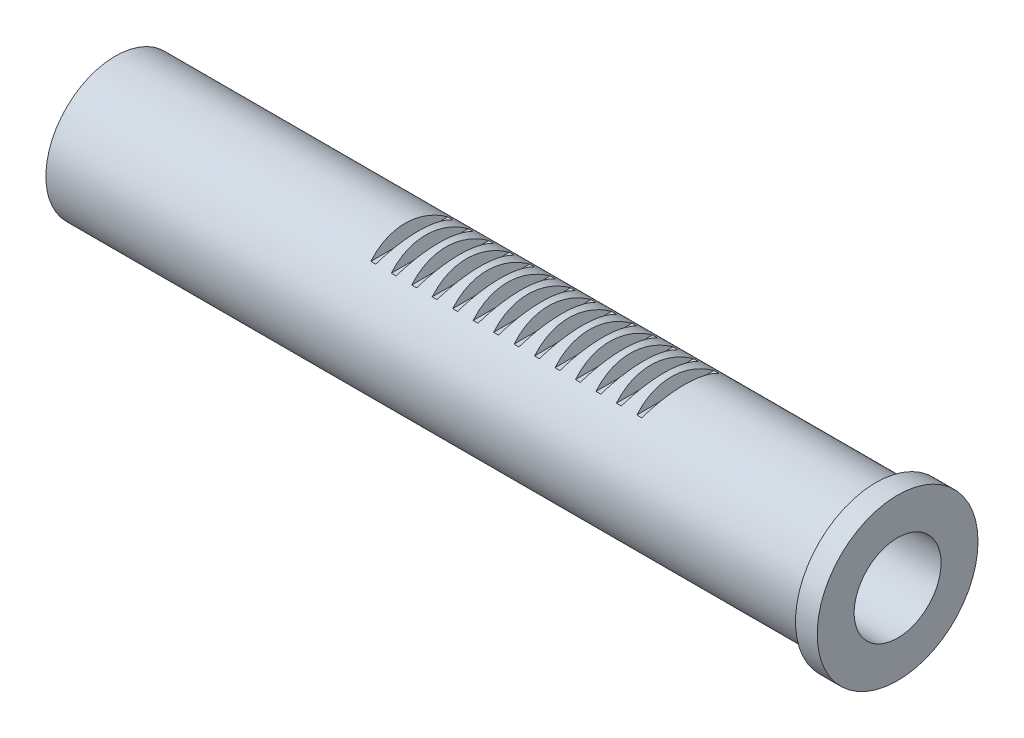
from build123d import *

# Parameters (mm, degrees)
SKETCH1_R               = 16
BOSS_EXTRUDE1_DEPTH     = 175
SKETCH2_R               = 18.5
BOSS_EXTRUDE2_DEPTH     = 5
SKETCH3_R               = 10
CUT_EXTRUDE1_DEPTH      = 100
SKETCH4_R               = 6
CUT_EXTRUDE2_DEPTH      = 8000
CUT_EXTRUDE3_DEPTH      = 182.891451146
CUT_EXTRUDE3_DEPTH_BACK = 182.891451146


with BuildPart() as part:
    # Sketch1 → Boss-Extrude1 (new body)
    with BuildSketch(Plane(origin=(0, 0, 0), x_dir=(0, 0, -1), z_dir=(1, 0, 0))):
        Circle(SKETCH1_R)
    extrude(amount=BOSS_EXTRUDE1_DEPTH)

    # Sketch2 → Boss-Extrude2 (add)
    with BuildSketch(Plane(origin=(175, 0, 0), x_dir=(0, 0, -1), z_dir=(1, 0, 0))):
        Circle(SKETCH2_R)
    extrude(amount=BOSS_EXTRUDE2_DEPTH)

    # Sketch3 → Cut-Extrude1 (cut)
    with BuildSketch(Plane(origin=(180, 0, 0), x_dir=(0, 0, -1), z_dir=(1, 0, 0))):
        Circle(SKETCH3_R)
    extrude(amount=-CUT_EXTRUDE1_DEPTH, mode=Mode.SUBTRACT)

    # Sketch4 → Cut-Extrude2 (cut)
    with BuildSketch(Plane(origin=(180, 0, 0), x_dir=(0, 0, -1), z_dir=(1, 0, 0))):
        Circle(SKETCH4_R)
    extrude(amount=-CUT_EXTRUDE2_DEPTH, mode=Mode.SUBTRACT)

    # Sketch5 → Cut-Revolve1 (revolve, cut)
    with BuildSketch(Plane.XY, mode=Mode.PRIVATE) as cut_revolve1_sk:
        Polygon((0, 0), (50, 0), (50, 6), (0, 11), align=None)
    revolve(cut_revolve1_sk.sketch.rotate(Axis((0, 0, 0), (1, 0, 0)), 270), axis=Axis((0, 0, 0), (1, 0, 0)), mode=Mode.SUBTRACT)

    # Sketch6 → Cut-Extrude3 (cut, two sides: drawn at the far end of the back side and taken through both)
    with BuildSketch(Plane.XY.offset(-CUT_EXTRUDE3_DEPTH_BACK)):
        Polygon((69.995219392, 16.697170081), (66.404780608, 16.697170081), (67.635, 13.317170081), (68.765, 13.317170081), align=None)
        Polygon((72.345, 13.317170081), (73.475, 13.317170081), (74.705219392, 16.697170081), (71.114780608, 16.697170081), align=None)
        Polygon((77.055, 13.317170081), (78.185, 13.317170081), (79.415219392, 16.697170081), (75.824780608, 16.697170081), align=None)
        Polygon((81.765, 13.317170081), (82.895, 13.317170081), (84.125219392, 16.697170081), (80.534780608, 16.697170081), align=None)
        Polygon((86.475, 13.317170081), (87.605, 13.317170081), (88.835219392, 16.697170081), (85.244780608, 16.697170081), align=None)
        Polygon((91.185, 13.317170081), (92.315, 13.317170081), (93.545219392, 16.697170081), (89.954780608, 16.697170081), align=None)
        Polygon((95.895, 13.317170081), (97.025, 13.317170081), (98.255219392, 16.697170081), (94.664780608, 16.697170081), align=None)
        Polygon((100.605, 13.317170081), (101.735, 13.317170081), (102.965219392, 16.697170081), (99.374780608, 16.697170081), align=None)
        Polygon((105.315, 13.317170081), (106.445, 13.317170081), (107.675219392, 16.697170081), (104.084780608, 16.697170081), align=None)
        Polygon((110.025, 13.317170081), (111.155, 13.317170081), (112.385219392, 16.697170081), (108.794780608, 16.697170081), align=None)
        Polygon((114.735, 13.317170081), (115.865, 13.317170081), (117.095219392, 16.697170081), (113.504780608, 16.697170081), align=None)
        Polygon((119.445, 13.317170081), (120.575, 13.317170081), (121.805219392, 16.697170081), (118.214780608, 16.697170081), align=None)
        Polygon((124.155, 13.317170081), (125.285, 13.317170081), (126.515219392, 16.697170081), (122.924780608, 16.697170081), align=None)
        Polygon((128.865, 13.317170081), (129.995, 13.317170081), (131.225219392, 16.697170081), (127.634780608, 16.697170081), align=None)
    extrude(amount=CUT_EXTRUDE3_DEPTH + CUT_EXTRUDE3_DEPTH_BACK, mode=Mode.SUBTRACT)


solid = part.part
